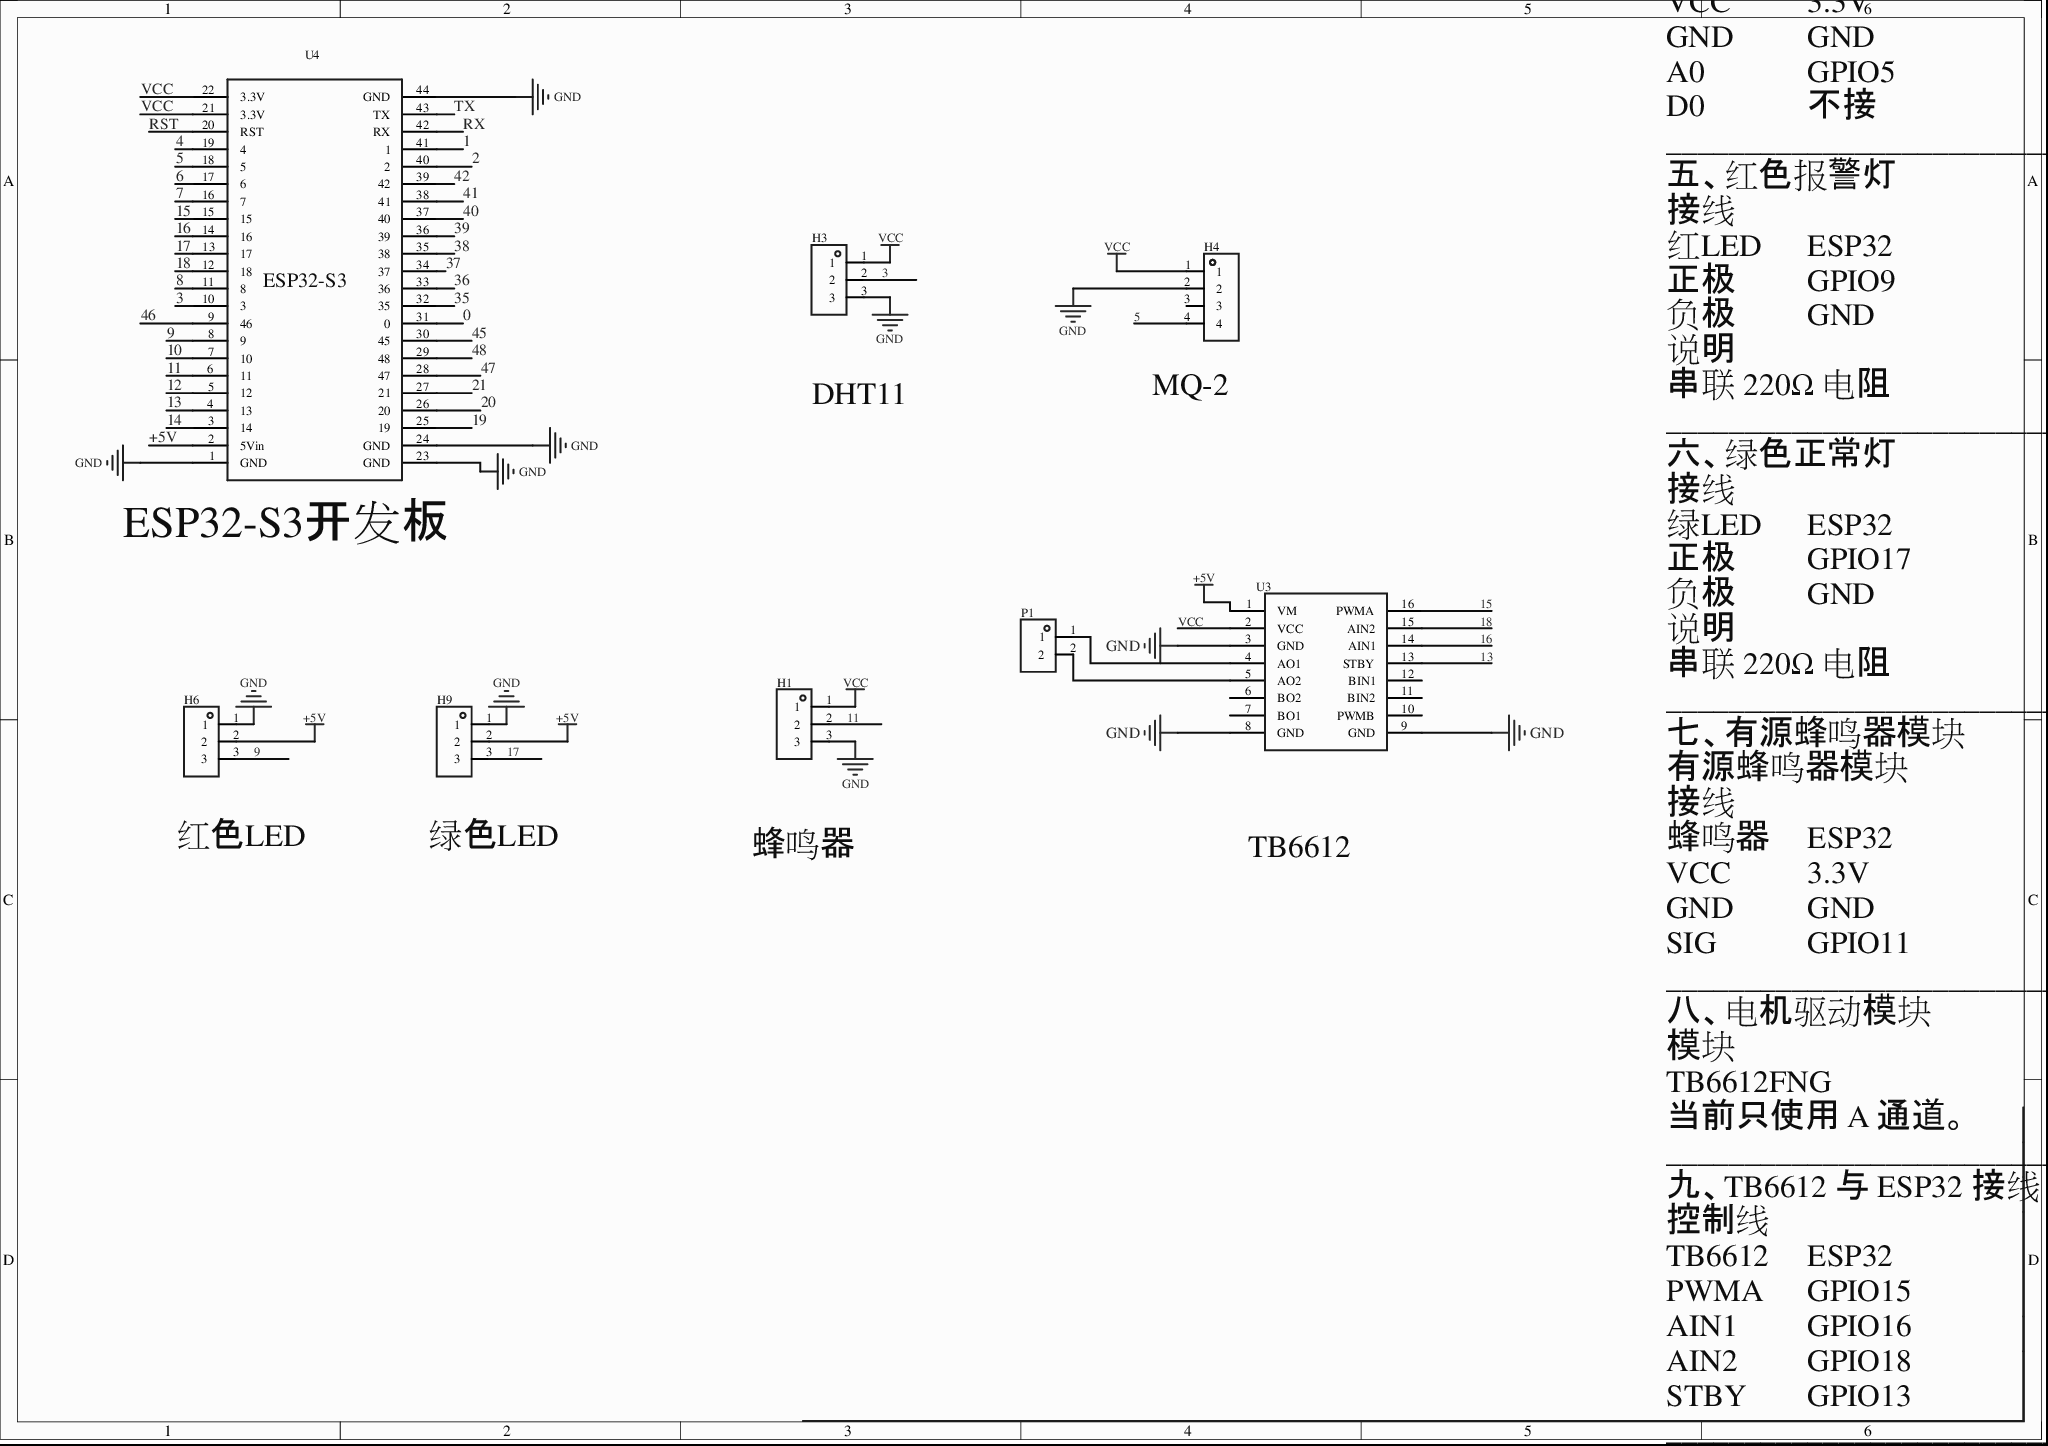
[diagram p0: MISC52005-3.schdoc]
# Altium project MISC52005-2.PrjPcb
1 sheet, 8 parts. Net scope: global (net labels, ports and power ports of the same name join across sheets).
Board file: MISC52005.pcbdoc

## Sheet MISC52005-3.schdoc
size 297 x 209 mm; Version: V1.0; @Project Name: MISC52005; @Page Count: 1; @Update Date: 2026-05-20; @Create Date: 2026-05-20; @Schematic Name: MISC52005; @Page No: 1; @Create Time: 23:22:16; @Update Time: 17:32:40; @Board Name: MISC52005

### Parts
H1  (no value)  [HDR-TH_3P-P2.54-V-F]
H3  (no value)  [HDR-TH_3P-P2.54-V-F]
H4  (no value)  [HDR-TH_4P-P2.54-V-F]
H6  (no value)  [HDR-TH_3P-P2.54-V-F]
H9  (no value)  [HDR-TH_3P-P2.54-V-F]
P1  KF301-2P接线端子  [CONN-TH_XY301V-A-5.0-2P]  (value not drawn)
U3  (no value)  [tb6612]
U4  NO  [ESP32S3]  (value not drawn)

### Nets
+5V: H6.2 H9.2 U3.1(VM) U4.2(5Vin)
GND: H1.3 H3.3 H4.2 H6.1 H9.1 U3.3(GND) U3.8(GND) U3.9(GND) U4.1(GND) U4.23(GND) U4.24(GND) U4.44(GND)
VCC: H1.1 H3.1 H4.1 U3.2(VCC) U4.21(3.3V) U4.22(3.3V)
0: U4.31(0)
1: U4.41(1)
2: U4.40(2)
3: H3.2 U4.10(3)
4: U4.19(4)
5: H4.4 U4.18(5)
6: U4.17(6)
7: U4.16(7)
8: U4.11(8)
9: H6.3 U4.8(9)
10: U4.7(10)
11: H1.2 U4.6(11)
12: U4.5(12)
13: U3.13(STBY) U4.4(13)
14: U4.3(14)
15: U3.16(PWMA) U4.15
16: U3.14(AIN1) U4.14(16)
17: H9.3 U4.13(17)
18: U3.15(AIN2) U4.12(18)
19: U4.25(19)
20: U4.26(20)
21: U4.27(21)
35: U4.32(35)
36: U4.33(36)
37: U4.34(37)
38: U4.35(38)
39: U4.36(39)
40: U4.37(40)
41: U4.38(41)
42: U4.39(42)
45: U4.30(45)
46: U4.9(46)
47: U4.28(47)
48: U4.29(48)
RST: U4.20(RST)
RX: U4.42(RX)
TX: U4.43(TX)
NetP1_1: P1.1 U3.4(AO1)
NetP1_2: P1.2 U3.5(AO2)

Not connected (* = marked no-connect by the designer): H4 3; U3 6(BO2) 7(BO1) 10(PWMB) 11(BIN2) 12(BIN1)

### Notes on the sheet
- 一、主控板
  主控
  ESP32-S3
  ________________________________________
  二、电源系统
  输入电源
  名称	规格
  USB Type-C	5V输入
  ________________________________________
  电源分配
  模块	电压
  ESP32-S3	USB 5V
  DHT11	3.3V
  MQ-2	3.3V
  TB6612逻辑	3.3V
  风机电机	5V
  LED	GPIO输出
  蜂鸣器	3.3V
  ________________________________________
  三、DHT11 温湿度模块
  DHT11
  接线
  DHT11	ESP32
  VCC	3.3V
  GND	GND
  DATA	GPIO3
  ________________________________________
  四、MQ-2 气体传感器模块
  MQ-2
  接线
  MQ-2	ESP32
  VCC	3.3V
  GND	GND
  A0	GPIO5
  D0	不接
  ________________________________________
  五、红色报警灯
  接线
  红LED	ESP32
  正极	GPIO9
  负极	GND
  说明
  串联 220Ω 电阻
  ________________________________________
  六、绿色正常灯
  接线
  绿LED	ESP32
  正极	GPIO17
  负极	GND
  说明
  串联 220Ω 电阻
  ________________________________________
  七、有源蜂鸣器模块
  有源蜂鸣器模块
  接线
  蜂鸣器	ESP32
  VCC	3.3V
  GND	GND
  SIG	GPIO11
  ________________________________________
  八、电机驱动模块
  模块
  TB6612FNG
  当前只使用 A 通道。
  ________________________________________
  九、TB6612 与 ESP32 接线
  控制线
  TB6612	ESP32
  PWMA	GPIO15
  AIN1	GPIO16
  AIN2	GPIO18
  STBY	GPIO13
  ________________________________________
  电源线
  TB6612	电源
  VM	5V
  VCC	3.3V
  GND	GND
  ________________________________________
  十、风机/电机接线
  风机
  5V直流风扇
  接线
  风机	TB6612
  正极	A01
  负极	A02
- DHT11
- (near H4) MQ-2
- (near U4) ESP32-S3开发板
- (near H6) 红色LED
- (near H9) 绿色LED
- 蜂鸣器
- TB6612

### Library data of the parts
H1 H3 H6 = HDR-F_2.54_1x3P: Symbol: PM254V-11-03-H85; ConvertToPcb: yes; ModelId: f3b3cc5aae9641bf9e56fc160cef875b; ModelName: HDR2.54-F-LI-1X3P; ModelTransform: 299.9994,100,0,0,0,0,0,0,-118.11; Device: HDR-F_2.54_1x3P; FootprintName: HDR-TH_3P-P2.54-V-F; AddInBom: yes; SupplierPart: C541850; Supplier Footprint: 插件
H4 = HDR-F_2.54_1x4P: Symbol: 2.54-1*4P母; ConvertToPcb: yes; ModelId: d187812051054f85879fcaa51a310d8e0819f05c4eef4c71ace90d822a990e87; ModelTransform: 419.6842,98.464,0,0,0,0,0,0,-118.11; Device: HDR-F_2.54_1x4P; FootprintName: HDR-TH_4P-P2.54-V-F; AddInBom: yes; SupplierPart: C2718488; Supplier Footprint: 插件; ModelName: HDR-TH_4P-P2.54-V-F
H9 = HDR-F_2.54_1x3P: Symbol: PM254V-11-03-H85; 3D Model: f3b3cc5aae9641bf9e56fc160cef875b; 3D Model Transform: 299.9994,100,0,0,0,0,0,0,-118.11; ConvertToPcb: yes; ModelName: HDR2.54-F-LI-1X3P; Device: HDR-F_2.54_1x3P; Supplier Part: C541850; Supplier Footprint: 插件; FootprintName: HDR-TH_3P-P2.54-V-F; AddInBom: yes
P1 = KF301-2P接线端子: 3D Model: ef7ead88b0f2448d904975b26718870f; 3D Model Transform: 417.322,299.212,0,0,0,0,11.811,-7.835,-157.48; AddInBom: yes; Symbol: KF301-2P接线端子; Device: KF301-2P接线端子; LCSC Part Name: KF301-2P接线端子; Supplier Part: C9900016950; Manufacturer Part: KF301-2P接线端子; Supplier Footprint: CK301-2P; Supplier: LCSC; ConvertToPcb: yes; FootprintName: CONN-TH_XY301V-A-5.0-2P; ModelName: CONN-TH_XY301V-A-5.0-2P
U3 = tb6612: AddInBom: yes; Symbol: tb6612; Device: tb6612; JLCPCB Part Class: 扩展库; ConvertToPcb: yes; FootprintName: tb6612
U4 = NO: Add into BOM: yes; Symbol: NO; Device: NO; Convert to PCB: yes; Origin Footprint: ESP32S3; FootprintName: ESP32S3